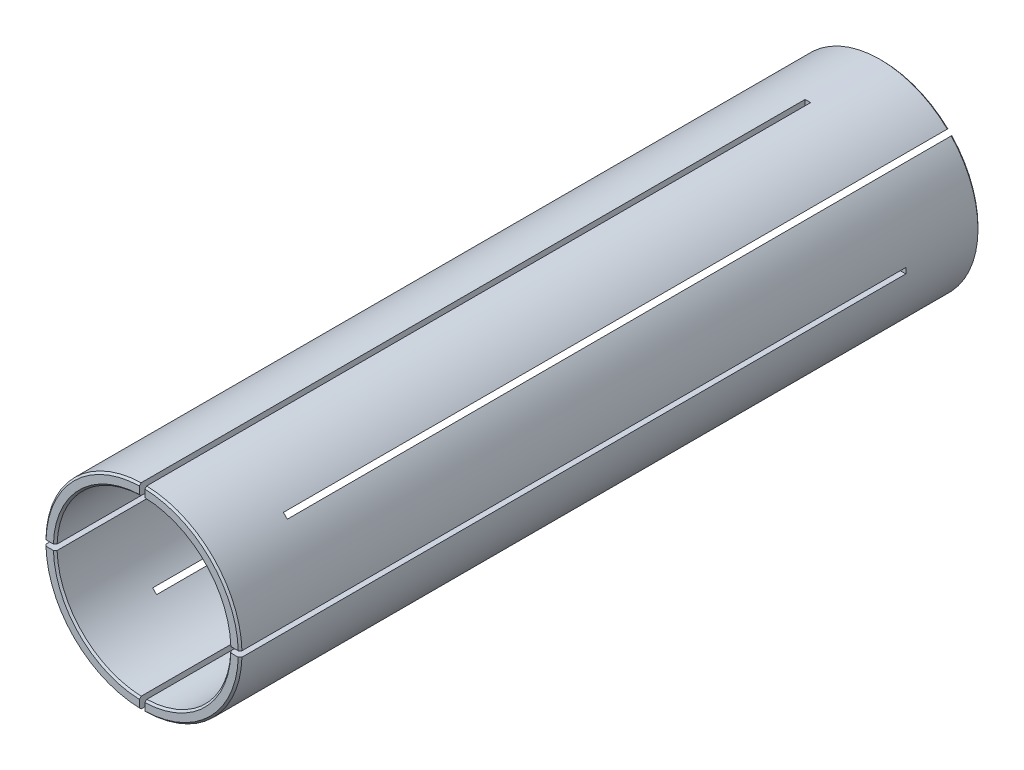
from build123d import *

# Parameters (mm, degrees)
SKETCH1_R           = 26.5
BOSS_EXTRUDE1_DEPTH = 200
SKETCH2_R           = 23.5
CUT_EXTRUDE1_DEPTH  = 200
CHAMFER1_SIZE       = 0.5
SKETCH4_W           = 1.5
SKETCH4_H           = 53
CUT_EXTRUDE2_DEPTH  = 180
CIRPATTERN1_COUNT   = 2
CIRPATTERN1_ANGLE   = 90
CUT_EXTRUDE3_DEPTH  = 180
CIRPATTERN2_COUNT   = 2
CIRPATTERN2_ANGLE   = 90


with BuildPart() as part:
    # Sketch1 → Boss-Extrude1 (new body)
    with BuildSketch(Plane.XY):
        Circle(SKETCH1_R)
    extrude(amount=BOSS_EXTRUDE1_DEPTH)

    # Sketch2 → Cut-Extrude1 (cut)
    with BuildSketch(Plane(origin=(0, 0, 0), x_dir=(-1, 0, 0), z_dir=(0, 0, -1))):
        Circle(SKETCH2_R)
    extrude(amount=-CUT_EXTRUDE1_DEPTH, mode=Mode.SUBTRACT)

    # Chamfer1
    chamfer1_edges = [part.edges().sort_by_distance(p)[0] for p in [
        (-26.5, 0, 0),
        (-26.5, 0, 200),
        (23.5, 0, 200),
        (23.5, 0, 0),
    ]]
    chamfer(chamfer1_edges, length=CHAMFER1_SIZE)

    # Sketch4 → Cut-Extrude2 (cut)
    with BuildSketch(Plane.XY.offset(200)):
        Rectangle(SKETCH4_W, SKETCH4_H)
    cut_extrude2 = extrude(amount=-CUT_EXTRUDE2_DEPTH, mode=Mode.SUBTRACT)

    # CirPattern1: Cut-Extrude2 ×2 about axis
    cirpattern1_axis = Axis((0, 0, 199.5), (0, 0, -1))
    for i in range(1, CIRPATTERN1_COUNT):
        add(cut_extrude2.rotate(cirpattern1_axis, i * CIRPATTERN1_ANGLE / (CIRPATTERN1_COUNT - 1)), mode=Mode.SUBTRACT)

    # Sketch5 → Cut-Extrude3 (cut)
    with BuildSketch(Plane(origin=(0, 0, 0), x_dir=(-1, 0, 0), z_dir=(0, 0, -1))):
        Polygon((-21.214455758, 20.159230222), (21.211951113, -22.267176649), (22.269893967, -21.209233795), (-20.156512904, 21.217173076), align=None)
    cut_extrude3 = extrude(amount=-CUT_EXTRUDE3_DEPTH, mode=Mode.SUBTRACT)

    # CirPattern2: Cut-Extrude3 ×2 about axis
    cirpattern2_axis = Axis((0, 0, 199.5), (0, 0, -1))
    for i in range(1, CIRPATTERN2_COUNT):
        add(cut_extrude3.rotate(cirpattern2_axis, i * CIRPATTERN2_ANGLE / (CIRPATTERN2_COUNT - 1)), mode=Mode.SUBTRACT)


solid = part.part
